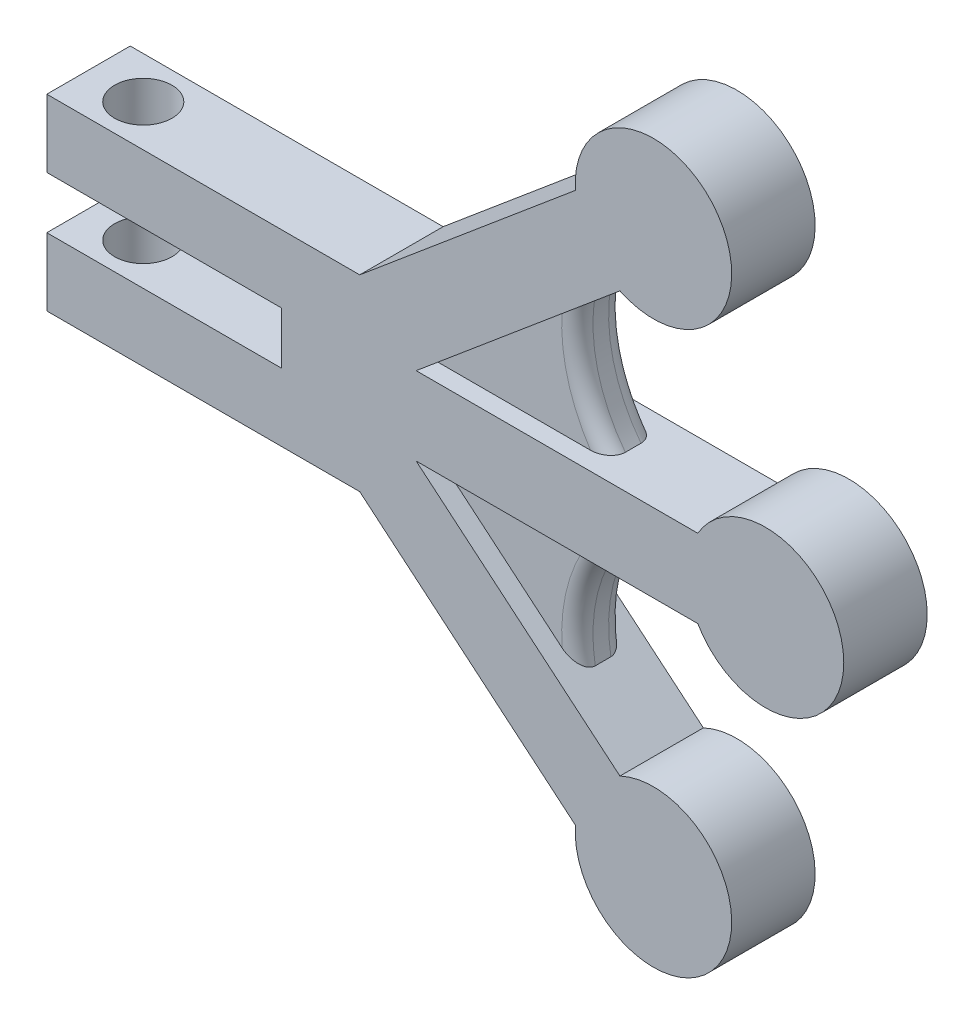
from build123d import *

# Parameters (mm, degrees)
SALIENTE_EXTRUIR1_DEPTH = 4
SALIENTE_EXTRUIR2_DEPTH = 1.5
CROQUIS3_W              = 15
CROQUIS3_H              = 4
CORTAR_EXTRUIR1_DEPTH   = 52.086410566
CROQUIS4_R              = 1.65
CORTAR_EXTRUIR2_DEPTH   = 54.601779767
FILLET2_R               = 1
SCALE1_SCALE            = 0.3
SKETCH2_R               = 15.04592303
CUT_EXTRUDE3_DEPTH      = 0.4
SKETCH3_R               = 13.988720819
CUT_EXTRUDE4_DEPTH      = 0.4
SKETCH4_W               = 4.5
SKETCH4_H               = 0.1
BOSS_EXTRUDE1_DEPTH     = 1.6
SKETCH5_R               = 0.55
CUT_EXTRUDE5_DEPTH      = 4.4


with BuildPart() as part:
    # Sketch1 → Saliente-Extruir1 (new, symmetric)
    with BuildSketch(Plane.XY):
        with BuildLine():
            Line((-6, 0), (-6, 6))
            Line((-6, 6), (14, 6))
            Line((14, 6), (27.788799976, 17.570176974))
            ThreePointArc((27.788799976, 17.570176974), (36.898130887, 20.772215113), (30.630237093, 13.427389365))
            Line((30.630237093, 13.427389365), (17.60748156, 2.5))
            Line((17.60748156, 2.5), (35.60748156, 2.5))
            ThreePointArc((35.60748156, 2.5), (44.937608579, 0), (35.60748156, -2.5))
            Line((35.60748156, -2.5), (17.60748156, -2.5))
            Line((17.60748156, -2.5), (30.630237093, -13.427389365))
            ThreePointArc((30.630237093, -13.427389365), (36.898130887, -20.772215113), (27.788799976, -17.570176974))
            Line((27.788799976, -17.570176974), (14, -6))
            Line((14, -6), (-6, -6))
            Line((-6, -6), (-6, 0))
        make_face()
    extrude(amount=SALIENTE_EXTRUIR1_DEPTH, both=True)

    # Croquis2 → Saliente-Extruir2 (add, symmetric)
    with BuildSketch(Plane.XY):
        with BuildLine():
            Line((26.884808669, 10.284601755), (14.628097579, 0))
            Line((14.628097579, 0), (26.884808669, -10.284601755))
            ThreePointArc((26.884808669, -10.284601755), (27.660138353, -4.406075759), (31.628097579, 0))
            ThreePointArc((31.628097579, 0), (27.660138353, 4.406075759), (26.884808669, 10.284601755))
        make_face()
    extrude(amount=SALIENTE_EXTRUIR2_DEPTH, both=True)

    # Croquis3 → Cortar-Extruir1 (cut, through all)
    with BuildSketch(Plane.XY.offset(4)):
        with Locations((1.5, 0)):
            Rectangle(CROQUIS3_W, CROQUIS3_H)
    extrude(amount=-CORTAR_EXTRUIR1_DEPTH, mode=Mode.SUBTRACT)

    # Croquis4 → Cortar-Extruir2 (cut, through all)
    with BuildSketch(Plane(origin=(0, 6, 0), x_dir=(1, 0, 0), z_dir=(0, 1, 0))):
        with Locations(Location((-2.5, 0, 0), (0, 0, 180))):
            Circle(CROQUIS4_R)
    extrude(amount=-CORTAR_EXTRUIR2_DEPTH, mode=Mode.SUBTRACT)

    # Fillet2
    fillet2_edges = [part.edges().sort_by_distance(p)[0] for p in [
        (27.034037659, -6.190607199, -1.5),
        (27.034037659, 6.190607199, -1.5),
        (27.034037659, -6.190607199, 1.5),
        (27.034037659, 6.190607199, 1.5),
    ]]
    fillet(fillet2_edges, radius=FILLET2_R)


with BuildPart() as part_1:
    # Scale1: scaled about (0, 0, 0)
    add(part.part.scale(SCALE1_SCALE))

    # Sketch2 → Cut-Extrude3 (cut)
    with BuildSketch(Plane.XY.offset(1.2)):
        Circle(SKETCH2_R)
    extrude(amount=-CUT_EXTRUDE3_DEPTH, mode=Mode.SUBTRACT)

    # Sketch3 → Cut-Extrude4 (cut)
    with BuildSketch(Plane(origin=(0, 0, -1.2), x_dir=(-1, 0, 0), z_dir=(0, 0, -1))):
        Circle(SKETCH3_R)
    extrude(amount=-CUT_EXTRUDE4_DEPTH, mode=Mode.SUBTRACT)

    # Sketch4 → Boss-Extrude1 (add)
    with BuildSketch(Plane.XY.offset(0.8)):
        with Locations((0.45, -0.55)):
            Rectangle(SKETCH4_W, SKETCH4_H)
        with Locations((0.45, 0.55)):
            Rectangle(SKETCH4_W, SKETCH4_H)
    extrude(amount=-BOSS_EXTRUDE1_DEPTH)

    # Sketch5 → Cut-Extrude5 (cut)
    with BuildSketch(Plane.XZ.offset(1.8)):
        with Locations((-0.75, 0)):
            Circle(SKETCH5_R)
    extrude(amount=-CUT_EXTRUDE5_DEPTH, mode=Mode.SUBTRACT)


solid = part_1.part
